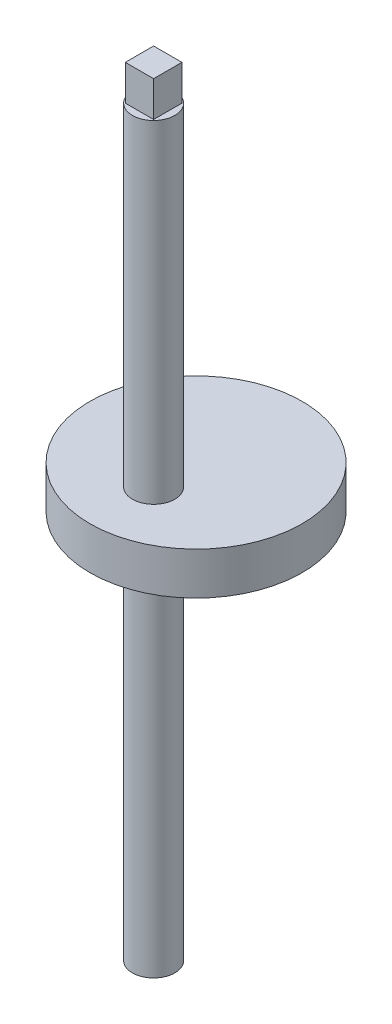
SolidWorks part; units mm, degrees
ref_plane "Front Plane" through (0, 0, 0) normal (0, 0, 1) x (1, 0, 0)
ref_plane "Top Plane" through (0, 0, 0) normal (0, 1, 0) x (1, 0, 0)
ref_plane "Right Plane" through (0, 0, 0) normal (1, 0, 0) x (0, 0, -1)
other "Configuration Table"
sketch "Sketch1" plane through (0, 0, 0) normal (0, 1, 0) x (1, 0, 0)
  circle A0 centre (0, 0) radius 15
  dimension "D1" = 30
extrude "Boss-Extrude1" add sketch "Sketch1" along normal mid plane 6
sketch "Sketch3" plane through (0, 0, 0) normal (0, 1, 0) x (1, 0, 0)
  circle A0 centre (0, -6) radius 3
  dimension "D1" = 6
  dimension "D2" = 6
extrude "Boss-Extrude2" add sketch "Sketch3" along normal mid plane 110
sketch "Sketch4" plane through (0, 55, 0) normal (0, 1, 0) x (1, 0, 0)
  line L1 (-2, -8) -> (2, -8)
  line L2 (-2, -8) -> (-2, -4)
  line L3 (-2, -4) -> (2, -4)
  line L4 (2, -8) -> (2, -4)
  line L5 (0, -4) -> (0, -8) construction
  line L6 (-2, -6) -> (2, -6) construction
  circle A0 centre (0, -6) radius 3 construction
  circle A1 centre (0, -6) radius 3
  dimension "D1" = 4
extrude "Cut-Extrude1" cut sketch "Sketch4" against normal blind 5
